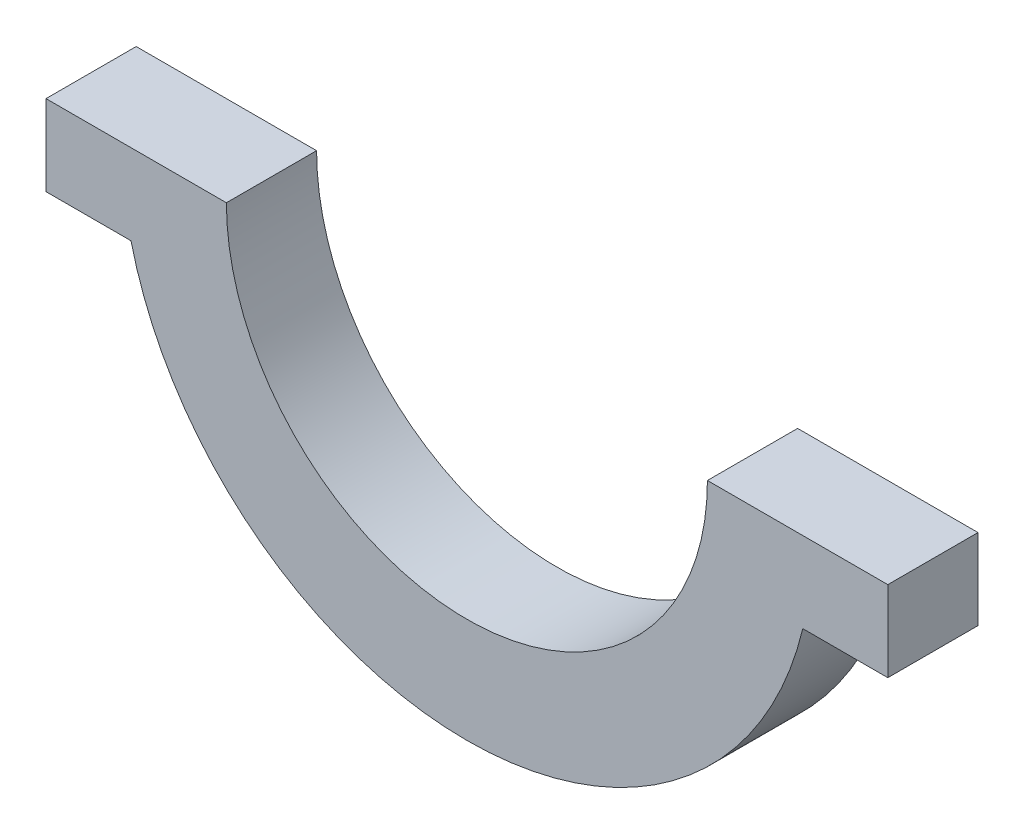
SolidWorks part; units mm, degrees
ref_plane "Front Plane" through (0, 0, 0) normal (0, 0, 1) x (1, 0, 0)
ref_plane "Top Plane" through (0, 0, 0) normal (0, 1, 0) x (1, 0, 0)
ref_plane "Right Plane" through (0, 0, 0) normal (1, 0, 0) x (0, 0, -1)
other "Configuration Table"
sketch "Sketch1" plane through (0, 0, 0) normal (0, 0, 1) x (1, 0, 0)
  line L0 (-16, 50) -> (-28, 50)
  line L1 (-28, 50) -> (-28, 44.6371)
  line L8 (28, 50) -> (28, 44.6371)
  line L9 (16, 50) -> (28, 50)
  line L10 (28, 44.6371) -> (22.3445, 44.6371)
  line L11 (-22.3445, 44.6371) -> (-28, 44.6371)
  arc A0 (-16, 50) -> (16, 50) centre (0, 50) ccw
  arc A1 (-22.3445, 44.6371) -> (22.3445, 44.6371) centre (0, 50) ccw
  dimension "D1" = 32
  dimension "D4" = 12
extrude "Boss-Extrude1" add sketch "Sketch1" along normal blind 6
